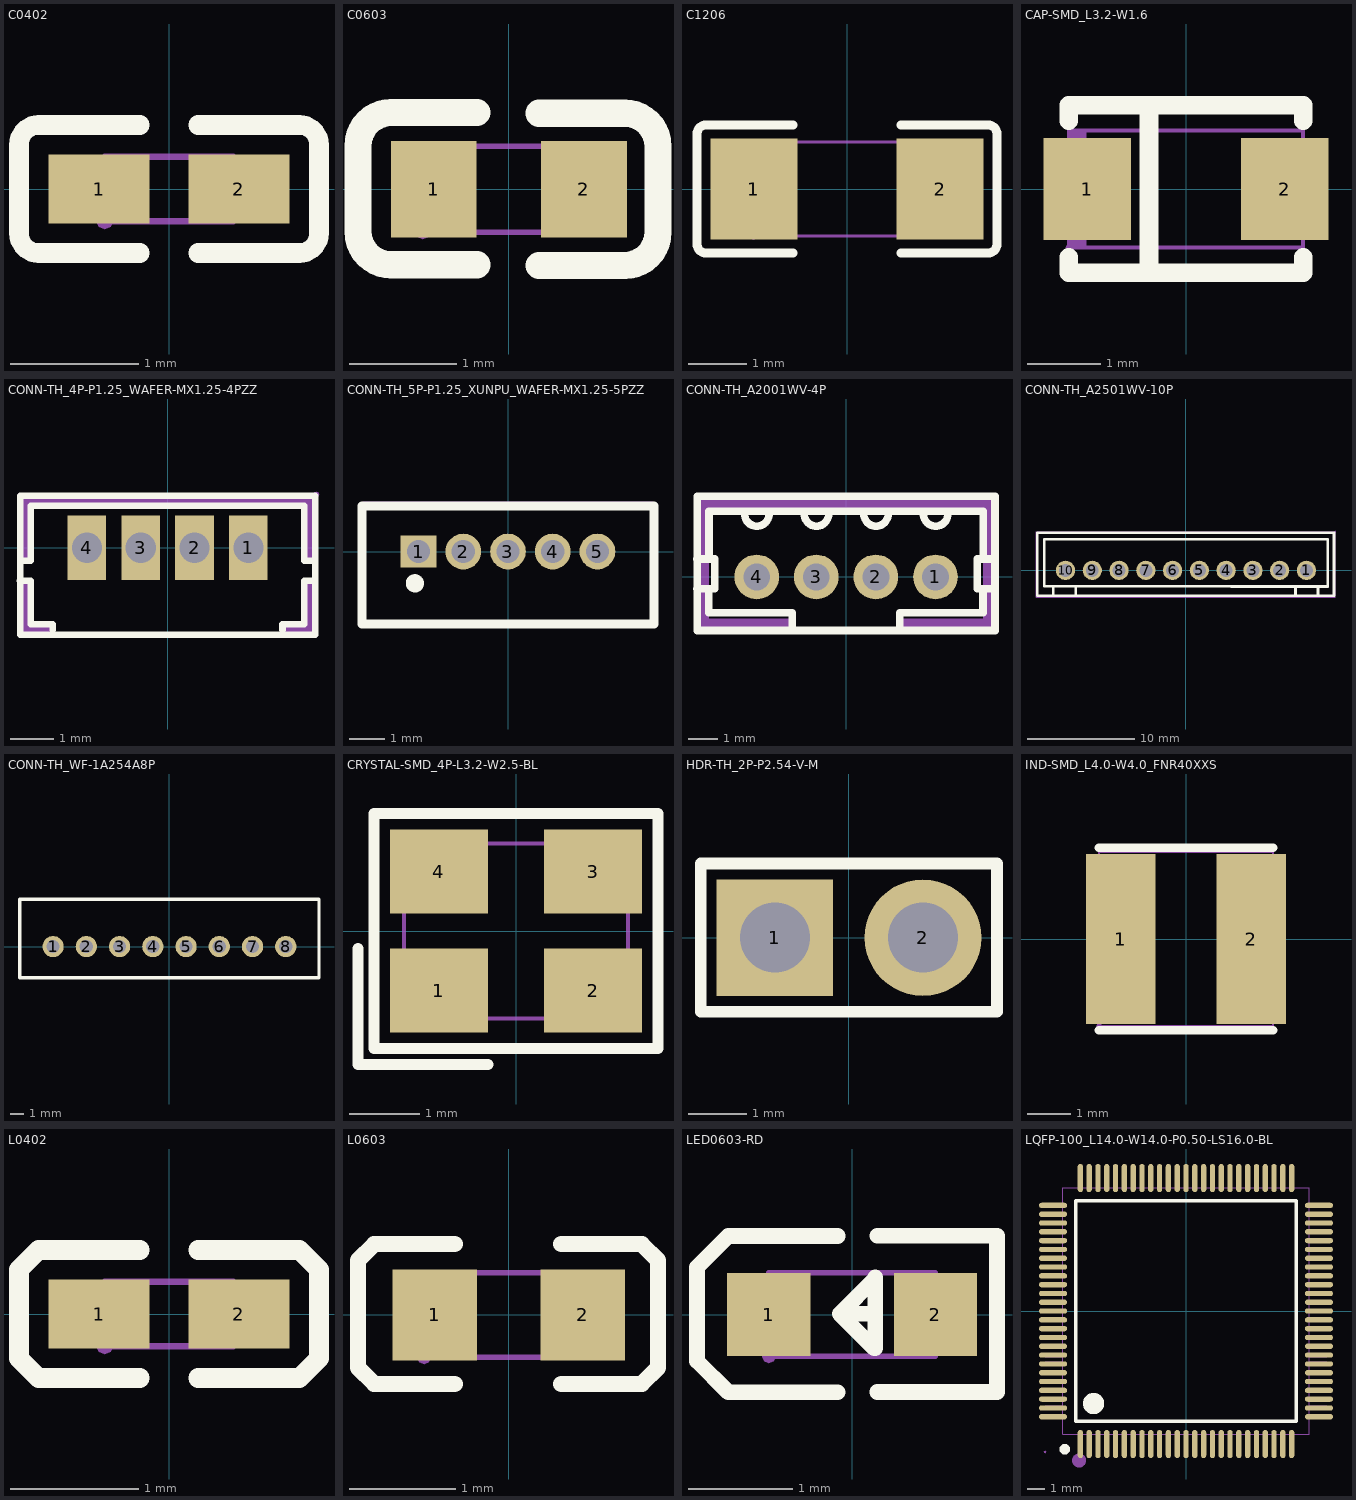
[diagram p0: the footprints below, top view; thin cyan lines are the x and y axes]
# Altium footprint library MISC86293-39.PcbLib: 27 footprints (part 1 of 2)
Each footprint in its own frame and in the unit in brackets; x right, y up, seen from the top. Pads: shape width x height; smd on the part's side, far side on the other; paste and mask are expansions set on the pad; w line width, h text height; cw(c..) or ccw(c..) is an arc to the next point about the centre after c.

## C0402 [mm]
pads (2):
  rect 0.79x0.54 smd paste-100 mask+0.051: 1(-0.545,0) 2(0.545,0)
Top Overlay:
  lines w0.152: -0.226,-0.499 -1.016,-0.499 cw(c-1.016,-0.346) -1.169,-0.346 -1.169,0.346 cw(c-1.016,0.346) -1.016,0.499 -0.226,0.499 ; 0.226,-0.499 1.016,-0.499 ccw(c1.016,-0.346) 1.169,-0.346 1.169,0.346 ccw(c1.016,0.346) 1.016,0.499 0.226,0.499
Top Paste:
  region: -0.18,0.225 -0.18,-0.225 -0.25,-0.275 -0.73,-0.275 -0.78,-0.225 -0.78,0.225 -0.73,0.275 -0.25,0.275
  region: 0.78,0.225 0.78,-0.225 0.73,-0.275 0.25,-0.275 0.18,-0.225 0.18,0.225 0.25,0.275 0.73,0.275
Mechanical 15:
  region: -0.5,-0.25 -0.5,0.25 -0.25,0.25 -0.25,-0.25
  region: 0.5,-0.25 0.5,0.25 0.25,0.25 0.25,-0.25
  region: -0.435,-0.25 -0.454,-0.296 -0.5,-0.315 -0.546,-0.296 -0.565,-0.25 -0.546,-0.204 -0.5,-0.185 -0.454,-0.204
  lines w0.051: -0.5,-0.25 -0.5,0.25 0.5,0.25 0.5,-0.25 -0.5,-0.25

## C0603 [mm]
pads (2):
  rect 0.8x0.9 smd: 1(-0.7,0) 2(0.7,0)
Top Overlay:
  lines w0.254: -0.296,-0.704 -1.096,-0.704 cw(c-1.096,-0.394) -1.406,-0.394 -1.405,0.406 cw(c-1.096,0.406) -1.096,0.715 -0.296,0.715 ; 0.28,-0.71 1.08,-0.71 ccw(c1.08,-0.4) 1.39,-0.4 1.39,0.4 ccw(c1.08,0.4) 1.08,0.71 0.28,0.71
Mechanical 15:
  region: -0.735,-0.4 -0.754,-0.446 -0.8,-0.465 -0.846,-0.446 -0.865,-0.4 -0.846,-0.354 -0.8,-0.335 -0.754,-0.354
  region: 0.8,-0.4 0.8,0.4 0.5,0.4 0.5,-0.4
  region: -0.8,-0.4 -0.8,0.4 -0.5,0.4 -0.5,-0.4
  lines w0.051: -0.8,-0.4 0.8,-0.4 0.8,0.4 -0.8,0.4 -0.8,-0.4

## C1206 [mm]
pads (2):
  rect 1.485x1.728 smd paste-100 mask+0.051: 1(-1.593,0) 2(1.593,0)
Top Overlay:
  lines w0.152: -0.926,-1.093 -2.411,-1.093 cw(c-2.411,-0.94) -2.564,-0.94 -2.564,0.94 cw(c-2.411,0.94) -2.411,1.093 -0.926,1.093 ; 0.926,-1.093 2.411,-1.093 ccw(c2.411,-0.94) 2.564,-0.94 2.564,0.94 ccw(c2.411,0.94) 2.411,1.093 0.926,1.093
Top Paste:
  region: -0.85,-0.764 -0.85,-0.394 -0.95,-0.294 -1.255,-0.294 -1.355,-0.194 -1.355,0.194 -1.255,0.294 -0.95,0.294 -0.85,0.394 -0.85,0.764 -0.95,0.864 -2.235,0.864 -2.335,0.764 -2.335,-0.764 -2.235,-0.864 -0.95,-0.864
  region: 0.85,-0.764 0.85,-0.394 0.95,-0.294 1.255,-0.294 1.355,-0.194 1.355,0.194 1.255,0.294 0.95,0.294 0.85,0.394 0.85,0.764 0.95,0.864 2.235,0.864 2.335,0.764 2.335,-0.764 2.235,-0.864 0.95,-0.864
Mechanical 15:
  region: 1.6,-0.8 1.6,0.8 1.1,0.8 1.1,-0.8
  region: -1.6,-0.8 -1.6,0.8 -1.1,0.8 -1.1,-0.8
  region: -1.535,-0.8 -1.554,-0.846 -1.6,-0.865 -1.646,-0.846 -1.665,-0.8 -1.646,-0.754 -1.6,-0.735 -1.554,-0.754
  lines w0.051: -1.6,-0.8 1.6,-0.8 1.6,0.8 -1.6,0.8 -1.6,-0.8

## CAP-SMD_L3.2-W1.6 [mm]
pads (2):
  rect 1.2x1.4 smd: 1(-1.35,0) 2(1.35,0)
Top Overlay:
  region: -0.635,1.143 -0.381,1.143 -0.381,-1.143 -0.635,-1.143
  lines w0.254: -1.6,-0.931 -1.6,-1.143 -0.128,-1.143 1.6,-1.143 1.6,-0.931 ; -1.6,0.931 -1.6,1.143 1.6,1.143 1.6,0.931
Mechanical 6:
  region: 1.48,0.06 1.48,-0.06 1,-0.06 1,0.06
  region: -1.48,0.06 -1.48,-0.06 -1,-0.06 -1,0.06
  region: -1.3,0.4 -1.3,-0.4 -1.18,-0.4 -1.18,0.4
  region: -1.6,0.8 -1.6,0.4 -1.36,0.4 -1.36,0.8
  region: -1.6,-0.8 -1.6,-0.4 -1.36,-0.4 -1.36,-0.8
Mechanical 15:
  region: -0.8,-0.6 -1.6,-0.6 -1.6,0.6 -0.8,0.6
  region: 0.8,0.6 1.6,0.6 1.6,-0.6 0.8,-0.6
  region: -1.557,-0.8 -1.569,-0.831 -1.6,-0.843 -1.631,-0.831 -1.643,-0.8 -1.631,-0.769 -1.6,-0.757 -1.569,-0.769
  lines w0.051: -1.6,-0.8 -1.6,0.8 1.6,0.8 1.6,-0.8 -1.6,-0.8

## CONN-TH_4P-P1.25_WAFER-MX1.25-4PZZ [mm]
pads (4):
  rect 0.9x1.5 hole 0.7 paste+0 mask+0.05: 1(1.875,0) 2(0.625,0) 3(-0.625,0) 4(-1.875,0)
Top Overlay:
  lines w0.152: -3.3,-0.3 -3.402,-0.3 -3.176,-0.3 -3.176,0.97 -0.001,0.97 3.174,0.97 3.174,-0.3 3.4,-0.3 3.299,-0.3 ; -2.668,-1.905 -2.668,-1.778 -3.176,-1.778 -3.176,-0.762 -3.303,-0.762 ; 2.667,-1.905 2.667,-1.778 3.175,-1.778 3.175,-0.762 3.302,-0.762 ; -3.303,-0.762 -3.43,-0.762 -3.303,-0.762 ; 3.302,-0.762 3.429,-0.762 3.302,-0.762 ; -3.42,-2.02 -3.42,1.21 3.43,1.21 3.43,-2.02 -3.42,-2.02
Mechanical 6:
  region: 2.665,-2.015 2.667,-1.778 3.175,-1.778 3.175,-0.762 3.429,-0.762 3.429,-2.015
  region: 3.4,1.2 3.4,-0.3 3.174,-0.3 3.174,0.97 0,0.97 0,1.22 3.43,1.22 3.43,1.2
  region: -2.665,-2.025 -2.667,-1.788 -3.175,-1.788 -3.175,-0.772 -3.429,-0.772 -3.429,-2.025
  region: -3.401,1.2 -3.401,-0.3 -3.174,-0.3 -3.174,0.97 0,0.97 0,1.22 -3.43,1.22 -3.43,1.2
Mechanical 15:
  region: -2.08,-0.15 -2.08,0.15 -1.67,0.15 -1.67,-0.15
  region: -0.83,-0.15 -0.83,0.15 -0.42,0.15 -0.42,-0.15
  region: 0.42,-0.15 0.42,0.15 0.83,0.15 0.83,-0.15
  region: 1.67,0.15 2.08,0.15 2.08,-0.15 1.67,-0.15
  region: 3.515,1.24 3.496,1.194 3.45,1.175 3.404,1.194 3.385,1.24 3.404,1.286 3.45,1.305 3.496,1.286
  lines w0.051: -3.45,-2.06 3.45,-2.06 3.45,1.24 -3.45,1.24 -3.45,-2.06

## CONN-TH_5P-P1.25_XUNPU_WAFER-MX1.25-5PZZ [mm]
pads (5):
  rect 1x0.9 hole 0.65: 1(-2.5,0)
  round 1 hole 0.65: 2(-1.25,0) 3(0,0) 4(1.25,0) 5(2.5,0)
Top Overlay:
  circle w0.254: c-2.601,-0.889 r0.127
  lines w0.254: -4.075,-2.03 4.075,-2.03 4.075,1.27 -4.075,1.27 -4.075,-2.03
Mechanical 6:
  region: -4.064,-1.778 -4.191,-1.778 -4.191,1.27 -4.064,1.397 4.064,1.397 4.191,1.27 4.191,-1.778 4.064,-1.778 4.064,1.143 3.937,1.27 -3.937,1.27 -4.064,1.143
Mechanical 15:
  region: -2.65,-0.205 -2.65,0.205 -2.35,0.205 -2.35,-0.205
  region: -1.4,0.205 -1.1,0.205 -1.1,-0.205 -1.4,-0.205
  region: -0.15,0.205 0.15,0.205 0.15,-0.205 -0.15,-0.205
  region: 1.1,0.205 1.4,0.205 1.4,-0.205 1.1,-0.205
  region: 2.35,0.205 2.65,0.205 2.65,-0.205 2.35,-0.205
  region: -4.01,-2.03 -4.029,-2.076 -4.075,-2.095 -4.121,-2.076 -4.14,-2.03 -4.121,-1.984 -4.075,-1.965 -4.029,-1.984
  lines w0.051: -4.075,-2.03 4.075,-2.03 4.075,1.27 -4.075,1.27 -4.075,-2.03

## CONN-TH_A2001WV-4P [mm]
pads (4):
  round 1.5 hole 0.9 paste+0 mask+0.05: 1(3,0) 2(1,0) 3(-1,0) 4(-3,0)
Top Overlay:
  lines w0.254: -5.002,-0.398 -4.402,-0.398 -4.402,0.602 -5.002,0.602 ; -4.602,-0.399 -4.602,-1.199 -1.801,-1.199 -1.801,-1.798 -0.203,-1.798 ; -4.6,0.8 -4.6,0.597 -4.6,2.202 4.6,2.202 4.6,0.602 ; -3.393,2.203 ccw(c-2.993,2.113) -2.593,2.203 ; -1.393,2.203 ccw(c-0.993,2.113) -0.593,2.203 ; 0.196,-1.796 1.801,-1.796 1.801,-1.196 4.595,-1.196 4.595,-0.396 ; 0.605,2.203 ccw(c1.005,2.113) 1.405,2.203 ; 2.605,2.203 ccw(c3.005,2.113) 3.405,2.203 ; 4.998,-1.798 4.998,2.702 ; 4.998,-0.398 4.398,-0.398 4.398,0.602 4.998,0.602 ; 5,-1.799 -5,-1.799 -5,2.702 5,2.702
Mechanical 6:
  region: 1.8,-1.8 5,-1.8 5,2.6 -5,2.6 -5,-1.8 -1.8,-1.8 -1.8,-1.4 -4.6,-1.4 -4.6,2.2 4.6,2.2 4.6,-1.4 1.8,-1.4
Mechanical 15:
  region: 5.065,-1.77 5.046,-1.816 5,-1.835 4.954,-1.816 4.935,-1.77 4.954,-1.724 5,-1.705 5.046,-1.724
  region: -2.745,0 -2.765,-0.098 -2.82,-0.18 -2.902,-0.235 -3,-0.255 -3.098,-0.235 -3.18,-0.18 -3.235,-0.098 -3.255,0 -3.235,0.098 -3.18,0.18 -3.098,0.235 -3,0.255 -2.902,0.235 -2.82,0.18 -2.765,0.098
  region: -0.745,0 -0.765,-0.098 -0.82,-0.18 -0.902,-0.235 -1,-0.255 -1.098,-0.235 -1.18,-0.18 -1.235,-0.098 -1.255,0 -1.235,0.098 -1.18,0.18 -1.098,0.235 -1,0.255 -0.902,0.235 -0.82,0.18 -0.765,0.098
  region: 1.255,0 1.235,-0.098 1.18,-0.18 1.098,-0.235 1,-0.255 0.902,-0.235 0.82,-0.18 0.765,-0.098 0.745,0 0.765,0.098 0.82,0.18 0.902,0.235 1,0.255 1.098,0.235 1.18,0.18 1.235,0.098
  region: 3.255,0 3.235,-0.098 3.18,-0.18 3.098,-0.235 3,-0.255 2.902,-0.235 2.82,-0.18 2.765,-0.098 2.745,0 2.765,0.098 2.82,0.18 2.902,0.235 3,0.255 3.098,0.235 3.18,0.18 3.235,0.098
  lines w0.051: -5,-1.8 -5,2.7 5,2.7 5,-1.8 -5,-1.8

## CONN-TH_A2501WV-10P [mm]
pads (10):
  round 1.8 hole 1.2: 1(11.25,0) 2(8.75,0) 3(6.25,0) 4(3.75,0) 5(1.25,0) 6(-1.25,0) 7(-3.75,0) 8(-6.25,0) 9(-8.75,0) 10(-11.25,0)
Top Overlay:
  lines w0.254: -13.883,-2.381 13.819,-2.381 ; -13.883,-2.378 -13.883,3.499 13.822,3.499 13.821,-2.381 ; -12.4,-2.284 -12.4,-1.484 ; -10.302,-2.3 -10.302,-1.5 ; 10.24,-2.3 10.24,-1.5 ; 12.338,-2.3 12.338,-1.5 ; 13.24,-1.5 13.24,2.9 -13.24,2.9 -13.24,-1.5 4.241,-1.5 13.241,-1.5
Mechanical 15:
  drawing of 15 lines, arcs and shapes, not listed

## CONN-TH_WF-1A254A8P [mm]
pads (8):
  round 1.6 hole 1: 1(-8.75,0) 2(-6.25,0) 3(-3.75,0) 4(-1.25,0) 5(1.25,0) 6(3.75,0) 7(6.25,0) 8(8.75,0)
Top Overlay:
  lines w0.254: -11.25,-2.35 11.25,-2.35 11.25,3.55 -11.25,3.55 -11.25,-2.35
Mechanical 15:
  region: -11.185,-2.35 -11.204,-2.396 -11.25,-2.415 -11.296,-2.396 -11.315,-2.35 -11.296,-2.304 -11.25,-2.285 -11.204,-2.304

## CRYSTAL-SMD_4P-L3.2-W2.5-BL [mm]
pads (4):
  rect 1.4x1.2 smd: 1(-1.1,-0.85) 2(1.1,-0.85) 3(1.1,0.85) 4(-1.1,0.85)
Top Overlay:
  lines w0.152: -2.257,-0.25 -2.257,-1.907 -0.4,-1.907 ; -2.029,-1.678 2.029,-1.678 2.029,1.679 -2.029,1.679 -2.029,-1.678
Mechanical 6:
  circle w0.254: c-1.27,-0.889 r0.127
Mechanical 15:
  region: -1.5,-0.35 -0.6,-0.35 -0.6,-1.15 -1.5,-1.15
  region: 0.6,-0.35 1.5,-0.35 1.5,-1.15 0.6,-1.15
  region: 0.6,1.15 1.5,1.15 1.5,0.35 0.6,0.35
  region: -1.5,1.15 -0.6,1.15 -0.6,0.35 -1.5,0.35
  region: -1.535,-1.25 -1.554,-1.296 -1.6,-1.315 -1.646,-1.296 -1.665,-1.25 -1.646,-1.204 -1.6,-1.185 -1.554,-1.204
  lines w0.051: -1.6,-1.25 1.6,-1.25 1.6,1.25 -1.6,1.25 -1.6,-1.25

## HDR-TH_2P-P2.54-V-M [mm]
pads (2):
  rect 2x2 hole 1.2: 1(-1.27,0)
  round 2 hole 1.2: 2(1.27,0)
Top Overlay:
  lines w0.203: -2.54,-1.27 -2.54,1.27 -0.635,1.27 2.54,1.27 2.54,-1.27 -2.54,-1.27
Mechanical 15:
  region: -1.59,0.32 -0.95,0.32 -0.95,-0.32 -1.59,-0.32
  region: 0.95,0.32 1.59,0.32 1.59,-0.32 0.95,-0.32
  region: -2.475,-1.25 -2.494,-1.296 -2.54,-1.315 -2.586,-1.296 -2.605,-1.25 -2.586,-1.204 -2.54,-1.185 -2.494,-1.204
  lines w0.051: -2.54,-1.25 2.54,-1.25 2.54,1.25 -2.54,1.25 -2.54,-1.25

## IND-SMD_L4.0-W4.0_FNR40XXS [mm]
pads (2):
  rect 1.6x3.9 smd: 1(-1.5,0) 2(1.5,0)
Top Overlay:
  lines w0.203: -2,-2.1 2,-2.1 ; -2,2.1 2,2.1
Mechanical 15:
  region: -1.051,1.65 -1.051,-1.65 -2.001,-1.65 -2.001,1.65
  region: 2.001,1.65 2.001,-1.65 1.051,-1.65 1.051,1.65
  region: -1.935,-2.003 -1.954,-2.049 -2,-2.068 -2.046,-2.049 -2.065,-2.003 -2.046,-1.957 -2,-1.938 -1.954,-1.957
  lines w0.051: -2,-2 2,-2 2,2 -2,2 -2,-2

## L0402 [mm]
pads (2):
  rect 0.79x0.54 smd paste-100 mask+0.051: 1(-0.545,0) 2(0.545,0)
Top Overlay:
  lines w0.152: -0.226,-0.499 -1.016,-0.499 -1.169,-0.346 -1.169,0.346 -1.016,0.499 -0.226,0.499 ; 0.226,-0.499 1.016,-0.499 1.169,-0.346 1.169,0.346 1.016,0.499 0.226,0.499
Top Paste:
  region: -0.135,-0.086 -0.135,0.086 -0.404,0.27 -0.9,0.27 -0.94,0.23 -0.94,-0.23 -0.9,-0.27 -0.404,-0.27
  region: 0.135,-0.086 0.135,0.086 0.404,0.27 0.9,0.27 0.94,0.23 0.94,-0.23 0.9,-0.27 0.404,-0.27
Mechanical 15:
  region: -0.435,-0.25 -0.454,-0.296 -0.5,-0.315 -0.546,-0.296 -0.565,-0.25 -0.546,-0.204 -0.5,-0.185 -0.454,-0.204
  region: 0.5,-0.25 0.5,0.25 0.25,0.25 0.25,-0.25
  region: -0.5,-0.25 -0.5,0.25 -0.25,0.25 -0.25,-0.25
  lines w0.051: -0.5,-0.25 0.5,-0.25 0.5,0.25 -0.5,0.25 -0.5,-0.25

## L0603 [mm]
pads (2):
  rect 0.8x0.864 smd paste-100 mask+0.051: 1(-0.7,0) 2(0.7,0)
Top Overlay:
  lines w0.152: -0.51,-0.651 -1.272,-0.651 -1.424,-0.499 -1.424,0.517 -1.272,0.67 -0.51,0.67 ; 0.496,-0.651 1.258,-0.651 1.411,-0.499 1.411,0.517 1.258,0.67 0.496,0.67
Top Paste:
  region: 0.264,0.154 0.264,-0.122 0.538,-0.416 1.042,-0.416 1.106,-0.352 1.106,0.384 1.042,0.448 0.538,0.448
  region: -0.252,0.143 -0.252,-0.134 -0.526,-0.427 -1.029,-0.427 -1.093,-0.363 -1.093,0.373 -1.029,0.437 -0.526,0.437
Mechanical 15:
  region: -0.735,-0.4 -0.754,-0.446 -0.8,-0.465 -0.846,-0.446 -0.865,-0.4 -0.846,-0.354 -0.8,-0.335 -0.754,-0.354
  region: -0.5,-0.4 -0.8,-0.4 -0.8,0.4 -0.5,0.4
  region: 0.8,-0.4 0.5,-0.4 0.5,0.4 0.8,0.4
  lines w0.051: -0.8,-0.4 -0.8,0.4 0.8,0.4 0.8,-0.4 -0.8,-0.4

## LED0603-RD [mm]
pads (2):
  rect 0.8x0.8 smd: 1(-0.799,0) 2(0.799,0)
Top Overlay:
  lines w0.15: -0.14,-0.746 -1.19,-0.746 -1.49,-0.446 -1.49,-0.346 -1.49,0.354 -1.49,0.454 -1.19,0.754 -0.14,0.754 ; 0.22,0.007 -0.12,0.007 ; 0.24,-0.744 1.39,-0.744 ; 0.24,0.757 1.39,0.757 1.39,-0.723 ; -0.12,0.007 0.22,0.347 0.22,0.357 0.22,-0.324 0.21,-0.324 -0.12,0.007
Mechanical 6:
  region: 0.529,0.068 1.069,0.068 1.069,-0.062 0.529,-0.062
  region: 0.735,-0.267 0.735,0.273 0.865,0.273 0.865,-0.267
  region: -1.07,0.062 -0.53,0.062 -0.53,-0.068 -1.07,-0.068
Mechanical 15:
  region: 0.5,-0.396 0.5,0.404 0.8,0.404 0.8,-0.396
  region: -0.8,-0.403 -0.8,0.397 -0.5,0.397 -0.5,-0.403
  region: -0.735,-0.403 -0.754,-0.449 -0.799,-0.468 -0.845,-0.449 -0.864,-0.403 -0.845,-0.358 -0.799,-0.339 -0.754,-0.358
  lines w0.051: -0.8,-0.4 0.8,-0.4 0.8,0.4 -0.8,0.4 -0.8,-0.4

## LQFP-100_L14.0-W14.0-P0.50-LS16.0-BL [mm]
pads (100):
  oval 0.3x1.6 smd paste-100 mask+0.051: 1(-6,-7.55) 2(-5.5,-7.55) 3(-5,-7.55) 4(-4.5,-7.55) 5(-4,-7.55) 6(-3.5,-7.55) 7(-3,-7.55) 8(-2.5,-7.55) 9(-2,-7.55) 10(-1.5,-7.55) 11(-1,-7.55) 12(-0.5,-7.55) 13(0,-7.55) 14(0.5,-7.55) 15(1,-7.55) 16(1.5,-7.55) 17(2,-7.55) 18(2.5,-7.55) 19(3,-7.55) 20(3.5,-7.55) 21(4,-7.55) 22(4.5,-7.55) 23(5,-7.55) 24(5.5,-7.55) 25(6,-7.55) 51(6,7.55) 52(5.5,7.55) 53(5,7.55) 54(4.5,7.55) 55(4,7.55) 56(3.5,7.55) 57(3,7.55) 58(2.5,7.55) 59(2,7.55) 60(1.5,7.55) 61(1,7.55) 62(0.5,7.55) 63(0,7.55) 64(-0.5,7.55) 65(-1,7.55) 66(-1.5,7.55) 67(-2,7.55) 68(-2.5,7.55) 69(-3,7.55) 70(-3.5,7.55) 71(-4,7.55) 72(-4.5,7.55) 73(-5,7.55) 74(-5.5,7.55) 75(-6,7.55)
  oval 1.6x0.3 smd paste-100 mask+0.051: 26(7.55,-6) 27(7.55,-5.5) 28(7.55,-5) 29(7.55,-4.5) 30(7.55,-4) 31(7.55,-3.5) 32(7.55,-3) 33(7.55,-2.5) 34(7.55,-2) 35(7.55,-1.5) 36(7.55,-1) 37(7.55,-0.5) 38(7.55,0) 39(7.55,0.5) 40(7.55,1) 41(7.55,1.5) 42(7.55,2) 43(7.55,2.5) 44(7.55,3) 45(7.55,3.5) 46(7.55,4) 47(7.55,4.5) 48(7.55,5) 49(7.55,5.5) 50(7.55,6) 76(-7.55,6) 77(-7.55,5.5) 78(-7.55,5) 79(-7.55,4.5) 80(-7.55,4) 81(-7.55,3.5) 82(-7.55,3) 83(-7.55,2.5) 84(-7.55,2) 85(-7.55,1.5) 86(-7.55,1) 87(-7.55,0.5) 88(-7.55,0) 89(-7.55,-0.5) 90(-7.55,-1) 91(-7.55,-1.5) 92(-7.55,-2) 93(-7.55,-2.5) 94(-7.55,-3) 95(-7.55,-3.5) 96(-7.55,-4) 97(-7.55,-4.5) 98(-7.55,-5) 99(-7.55,-5.5) 100(-7.55,-6)
Top Overlay:
  lines w0.2: -6.25,-6.25 -6.25,6.25 6.25,6.25 6.25,-6.25 -6.25,-6.25
  lines w0.3: -6.883,-7.696 ccw(c-6.882,-7.846) -6.881,-7.696
  lines w0.6: -5.25,-4.95 ccw(c-5.248,-5.25) -5.245,-4.95
Top Paste:
  drawing of 100 lines, arcs and shapes, not listed
Mechanical 6:
  circle w0.4: c-6.071,-8.484 r0.2
Mechanical 15:
  drawing of 205 lines, arcs and shapes, not listed